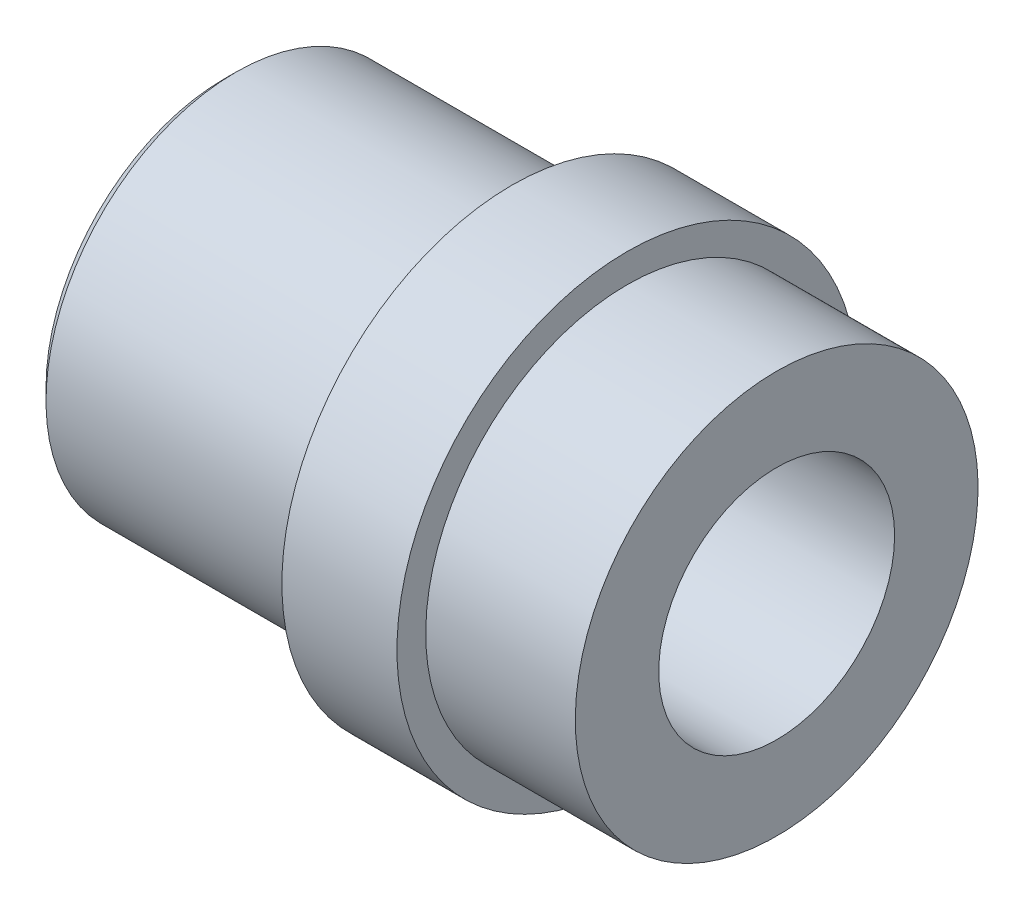
from build123d import *

# Parameters (mm, degrees)
SKETCH2_R                  = 10
CUT_EXTRUDE1_DEPTH         = 56.713553109
M22X1_5_TAPPED_HOLE2_D     = 20.5
M22X1_5_TAPPED_HOLE2_DEPTH = 22
M22X1_5_TAPPED_HOLE2_TIP   = 6.158821345


with BuildPart() as part:
    # Sketch1 → Revolve1 (revolve)
    with BuildSketch(Plane.XY):
        Polygon((-48, 0), (-48, 15.5), (-47, 16.5), (-23, 16.5), (-23, 20), (-13, 20), (-13, 17.5), (0, 17.5), (0, 0), align=None)
    revolve(axis=Axis((0, 0, 0), (-1, 0, 0)))

    # Sketch2 → Cut-Extrude1 (cut, through all)
    with BuildSketch(Plane(origin=(0, 0, 0), x_dir=(0, 0, -1), z_dir=(1, 0, 0))):
        with Locations(Location((0, 0, 0), (0, 0, 90))):
            Circle(SKETCH2_R)
    extrude(amount=-CUT_EXTRUDE1_DEPTH, mode=Mode.SUBTRACT)

    # M22x1.5 Tapped Hole2
    with Locations(Plane(origin=(0, 0, 0), x_dir=(0, 0, -1), z_dir=(1, 0, 0))):
        with Locations((0, 0)):
            Hole(M22X1_5_TAPPED_HOLE2_D / 2, depth=M22X1_5_TAPPED_HOLE2_DEPTH)
            with Locations((0, 0, -(M22X1_5_TAPPED_HOLE2_DEPTH + M22X1_5_TAPPED_HOLE2_TIP / 2))):  # 118° drill point
                Cone(0, M22X1_5_TAPPED_HOLE2_D / 2, M22X1_5_TAPPED_HOLE2_TIP, mode=Mode.SUBTRACT)


solid = part.part
